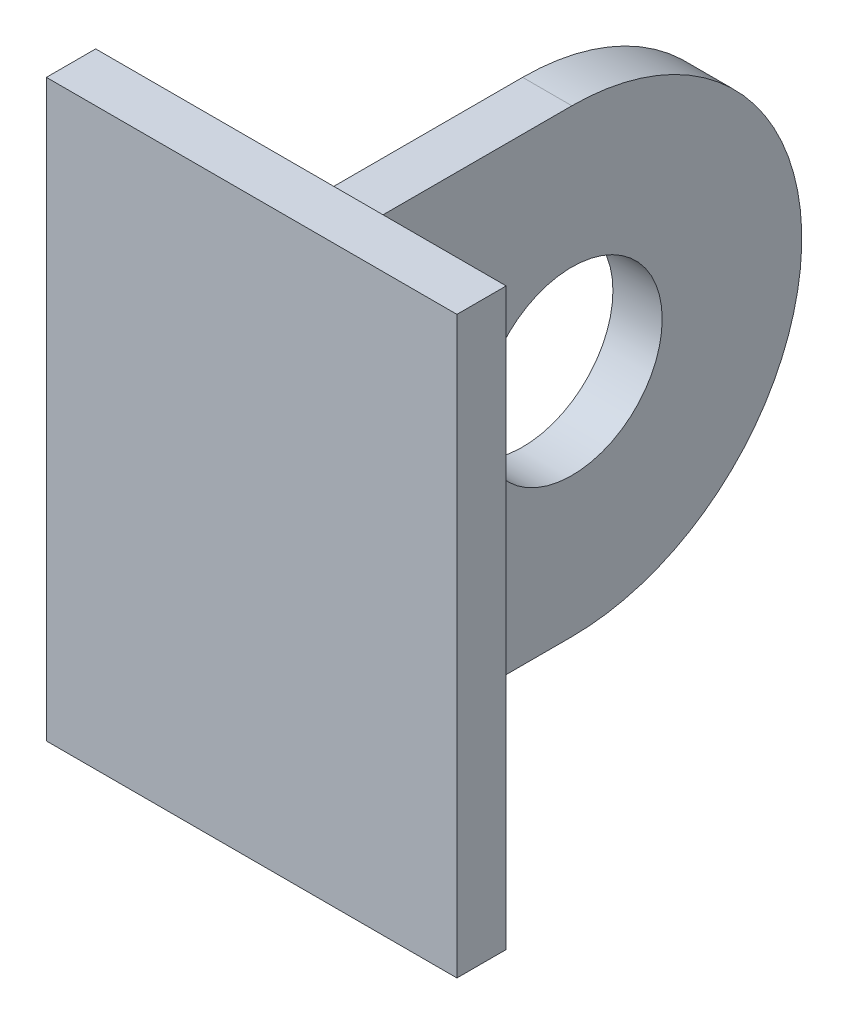
from build123d import *

# Parameters (mm, degrees)
SKETCH_1_W      = 25
SKETCH_1_H      = 35
EXTRUDE_1_DEPTH = 3
SKETCH_2_R      = 5.5
EXTRUDE_2_DEPTH = 1.5


with BuildPart() as part:
    # 草图1 → 凸台-拉伸1 (new body)
    with BuildSketch(Plane.XY):
        Rectangle(SKETCH_1_W, SKETCH_1_H)
    extrude(amount=EXTRUDE_1_DEPTH)


with BuildPart() as body_2:
    # 草图2 → 凸台-拉伸2 (new, symmetric)
    with BuildSketch(Plane(origin=(0, 0, 0), x_dir=(0, 0, -1), z_dir=(1, 0, 0))):
        with BuildLine():
            Line((0, 14), (15, 14))
            ThreePointArc((15, 14), (29, 0), (15, -14))
            Line((15, -14), (0, -14))
            Line((0, -14), (0, 14))
        make_face()
        with Locations((15, 0)):
            Circle(SKETCH_2_R, mode=Mode.SUBTRACT)
    extrude(amount=EXTRUDE_2_DEPTH, both=True)


solid = Compound([part.part, body_2.part])
